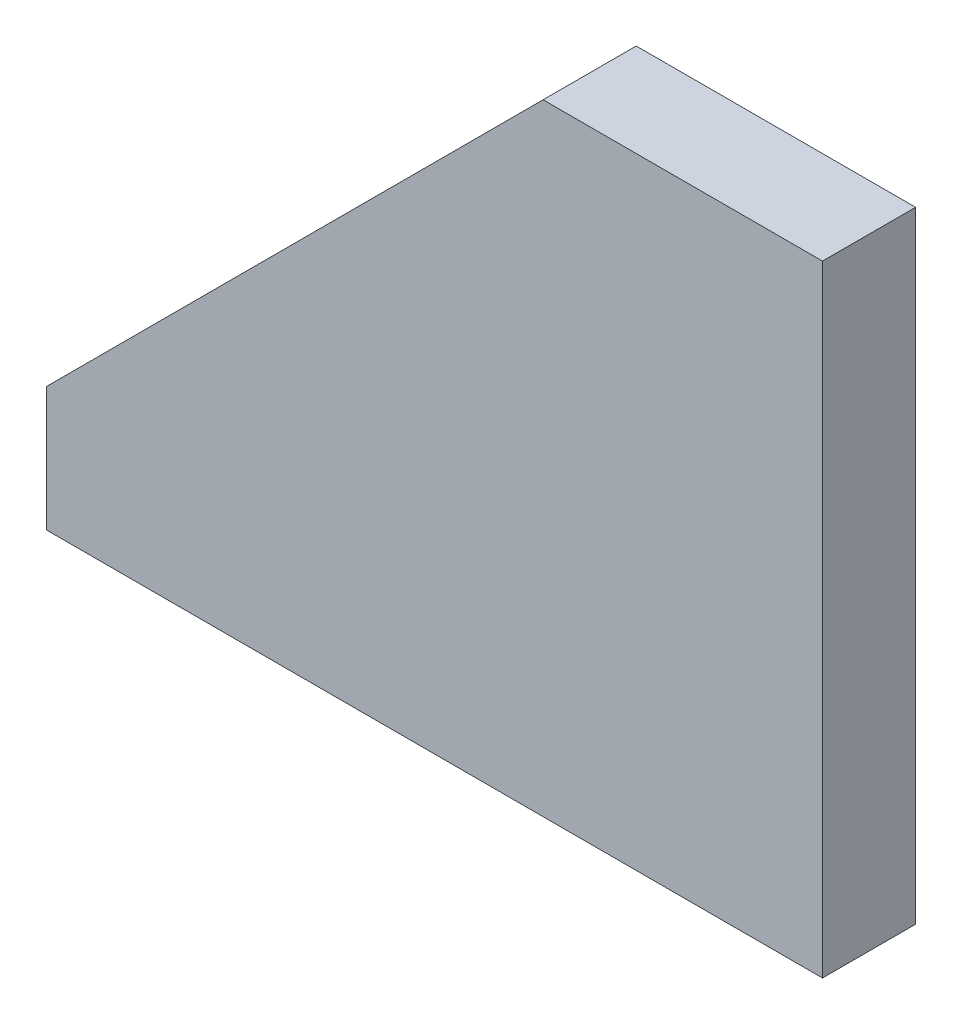
from build123d import *

# Parameters (mm, degrees)
SKETCH_1_W      = 125
SKETCH_1_H      = 100
EXTRUDE_1_DEPTH = 15
CHAMFER_1_SIZE  = 80


with BuildPart() as part:
    # 草图1 → 凸台-拉伸1 (new body)
    with BuildSketch(Plane.XY):
        Rectangle(SKETCH_1_W, SKETCH_1_H)
    extrude(amount=EXTRUDE_1_DEPTH)

    # 倒角1
    chamfer_1_edges = [part.edges().sort_by_distance(p)[0] for p in [
        (-62.5, 50, 7.5),
    ]]
    chamfer(chamfer_1_edges, length=CHAMFER_1_SIZE)


solid = part.part
